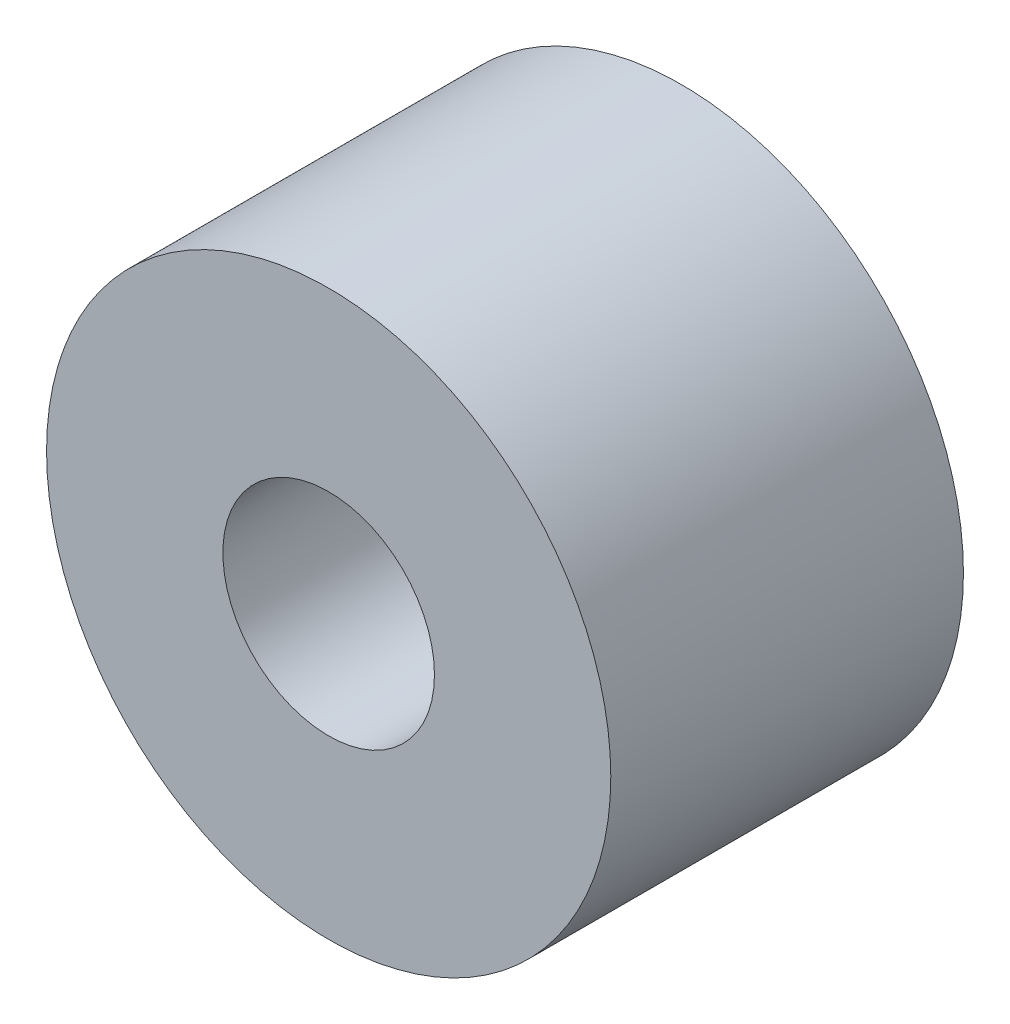
SolidWorks part; units mm, degrees
ref_plane "前视基准面" through (0, 0, 0) normal (0, 0, 1) x (1, 0, 0)
ref_plane "上视基准面" through (0, 0, 0) normal (0, 1, 0) x (1, 0, 0)
ref_plane "右视基准面" through (0, 0, 0) normal (1, 0, 0) x (0, 0, -1)
sketch "草图1" plane through (0, 0, 0) normal (0, 0, 1) x (1, 0, 0)
  circle A0 centre (0, 0) radius 40
  circle A1 centre (0, 0) radius 15
  dimension "D1" = 80
  dimension "D2" = 30
extrude "凸台-拉伸1" add sketch "草图1" along normal blind 50
